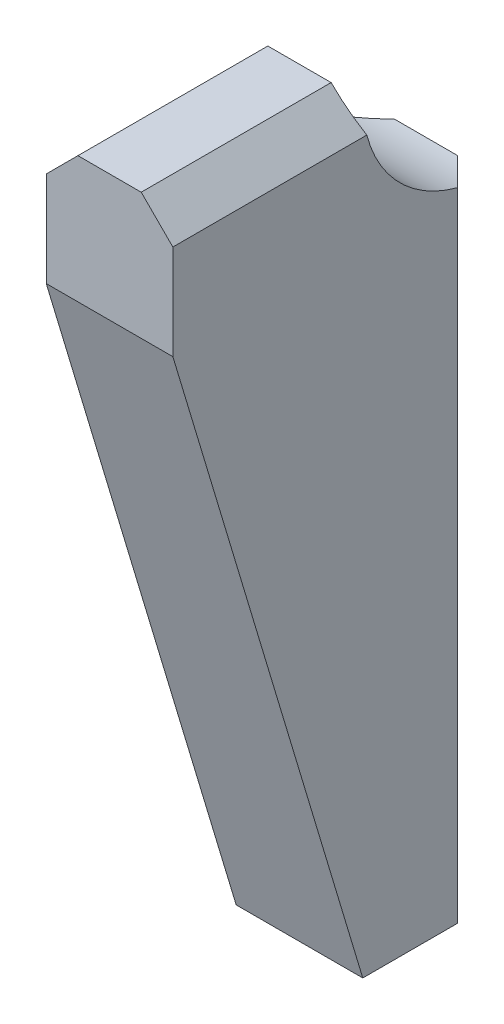
from build123d import *

# Parameters (mm, degrees)
BOSS_EXTRUDE1_DEPTH = 20
CHAMFER1_SIZE       = 10


with BuildPart() as part:
    # Sketch1 → Boss-Extrude1 (new, symmetric)
    with BuildSketch(Plane(origin=(0, 0, 0), x_dir=(0, 0, -1), z_dir=(1, 0, 0))):
        with BuildLine():
            Line((0, 0), (0, 200))
            ThreePointArc((0, 200), (-28.284271247, 211.715728753), (-40, 240))
            Line((-40, 240), (-100, 240))
            Line((-100, 240), (-100, 200))
            Line((-100, 200), (-40, 0))
            Line((-40, 0), (0, 0))
        make_face()
    extrude(amount=BOSS_EXTRUDE1_DEPTH, both=True)

    # Chamfer1
    chamfer1_edges = [part.edges().sort_by_distance(p)[0] for p in [
        (20, 240, 70),
        (-20, 240, 70),
        (20, 100, 0),
        (-20, 100, 0),
    ]]
    chamfer(chamfer1_edges, length=CHAMFER1_SIZE)


solid = part.part
